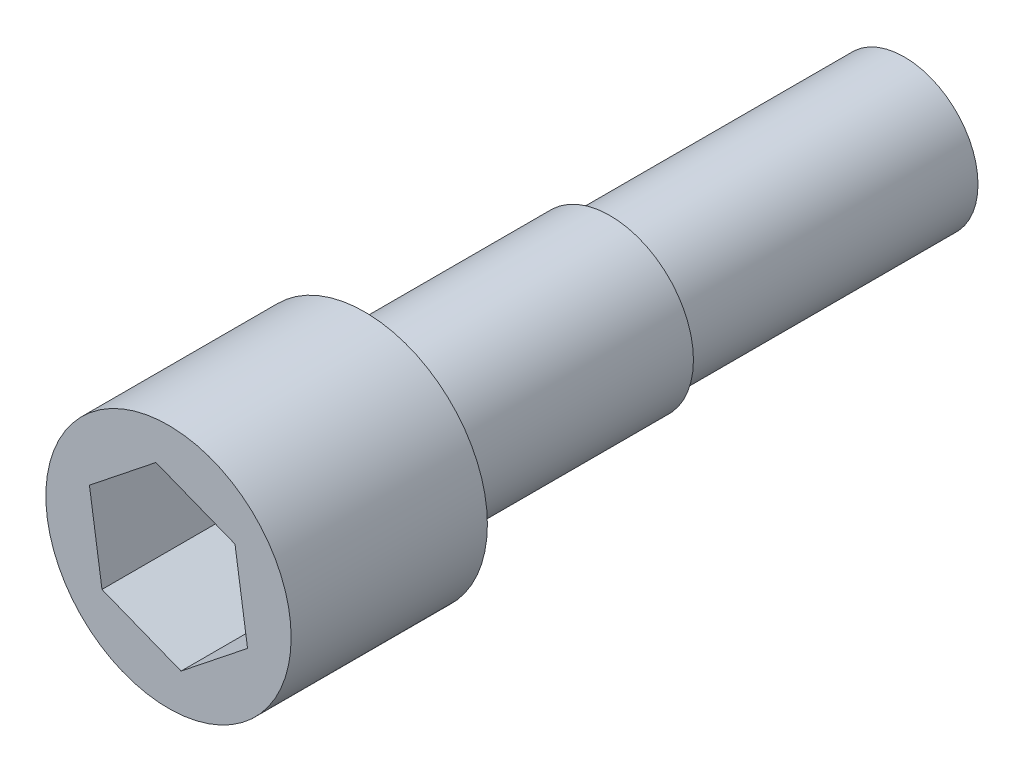
SolidWorks part; units mm, degrees
ref_plane "前视基准面" through (0, 0, 0) normal (0, 0, 1) x (1, 0, 0)
ref_plane "上视基准面" through (0, 0, 0) normal (0, 1, 0) x (1, 0, 0)
ref_plane "右视基准面" through (0, 0, 0) normal (1, 0, 0) x (0, 0, -1)
sketch "草图1" plane through (0, 0, 0) normal (0, 0, 1) x (1, 0, 0)
  circle A0 centre (0, -6) radius 1.7
  dimension "D1" = 3.4
extrude "凸台-拉伸1" add sketch "草图1" against normal blind 5
sketch "草图2" plane through (0, 0, -5) normal (0, 0, -1) x (-1, 0, 0)
  circle A0 centre (0, -6) radius 1.5
  dimension "D1" = 3
extrude "凸台-拉伸2" add sketch "草图2" along normal blind 6
sketch "草图3" plane through (0, 0, 0) normal (0, 0, 1) x (1, 0, 0)
  circle A0 centre (0, -6) radius 2.5
  dimension "D1" = 5
extrude "凸台-拉伸3" add sketch "草图3" along normal blind 4
sketch "草图4" plane through (0, 0, 4) normal (0, 0, 1) x (1, 0, 0)
  line L1 (1.3556, -4.9218) -> (-0.256, -4.287)
  line L2 (-0.256, -4.287) -> (-1.6115, -5.3651)
  line L3 (-1.6115, -5.3651) -> (-1.3556, -7.0782)
  line L4 (-1.3556, -7.0782) -> (0.256, -7.713)
  line L5 (0.256, -7.713) -> (1.6115, -6.6349)
  line L6 (1.6115, -6.6349) -> (1.3556, -4.9218)
  circle A0 centre (0, -6) radius 1.5 construction
  dimension "D1" = 3
extrude "切除-拉伸1" cut sketch "草图4" against normal blind 3
sketch "草图5" plane through (0, 0, 0) normal (0, 0, -1) x (-1, 0, 0)
  point P0 (0, -6)
